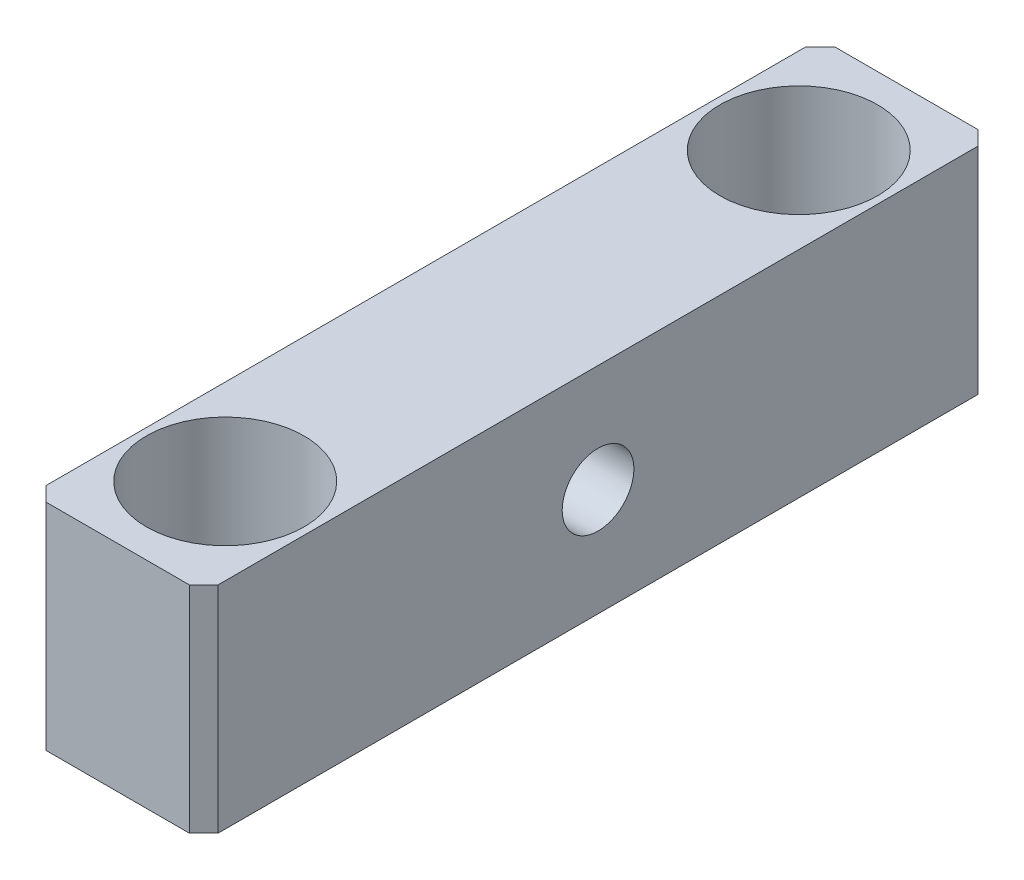
from build123d import *

# Parameters (mm, degrees)
SKETCH_1_W                   = 12
SKETCH_1_H                   = 55
EXTRUDE_1_DEPTH              = 7.5
CHAMFER_1_SIZE               = 1
HOLE_WIZARD_M6_1_D           = 6.6
HOLE_WIZARD_M6_1_CBORE_D     = 11
HOLE_WIZARD_M6_1_CBORE_DEPTH = 8
HOLE_WIZARD_M6_1_2_D         = 5


with BuildPart() as part:
    # 草图1 → 凸台-拉伸1 (new, symmetric)
    with BuildSketch(Plane(origin=(0, 0, 0), x_dir=(1, 0, 0), z_dir=(0, 1, 0))):
        Rectangle(SKETCH_1_W, SKETCH_1_H)
    extrude(amount=EXTRUDE_1_DEPTH, both=True)

    # 倒角1
    chamfer_1_edges = [part.edges().sort_by_distance(p)[0] for p in [
        (6, 0, 27.5),
        (-6, 0, 27.5),
        (-6, 0, -27.5),
        (6, 0, -27.5),
    ]]
    chamfer(chamfer_1_edges, length=CHAMFER_1_SIZE)

    # Hole Wizard M6 _1 (through all)
    with Locations(Plane(origin=(0, 7.5, 0), x_dir=(1, 0, 0), z_dir=(0, 1, 0))):
        with Locations((0, 20), (0, -20)):
            CounterBoreHole(HOLE_WIZARD_M6_1_D / 2, HOLE_WIZARD_M6_1_CBORE_D / 2, HOLE_WIZARD_M6_1_CBORE_DEPTH)

    # Hole Wizard M6 _1 2 (through all)
    with Locations(Plane.ZY.offset(6)):
        with Locations((0, 0)):
            Hole(HOLE_WIZARD_M6_1_2_D / 2)


solid = part.part
